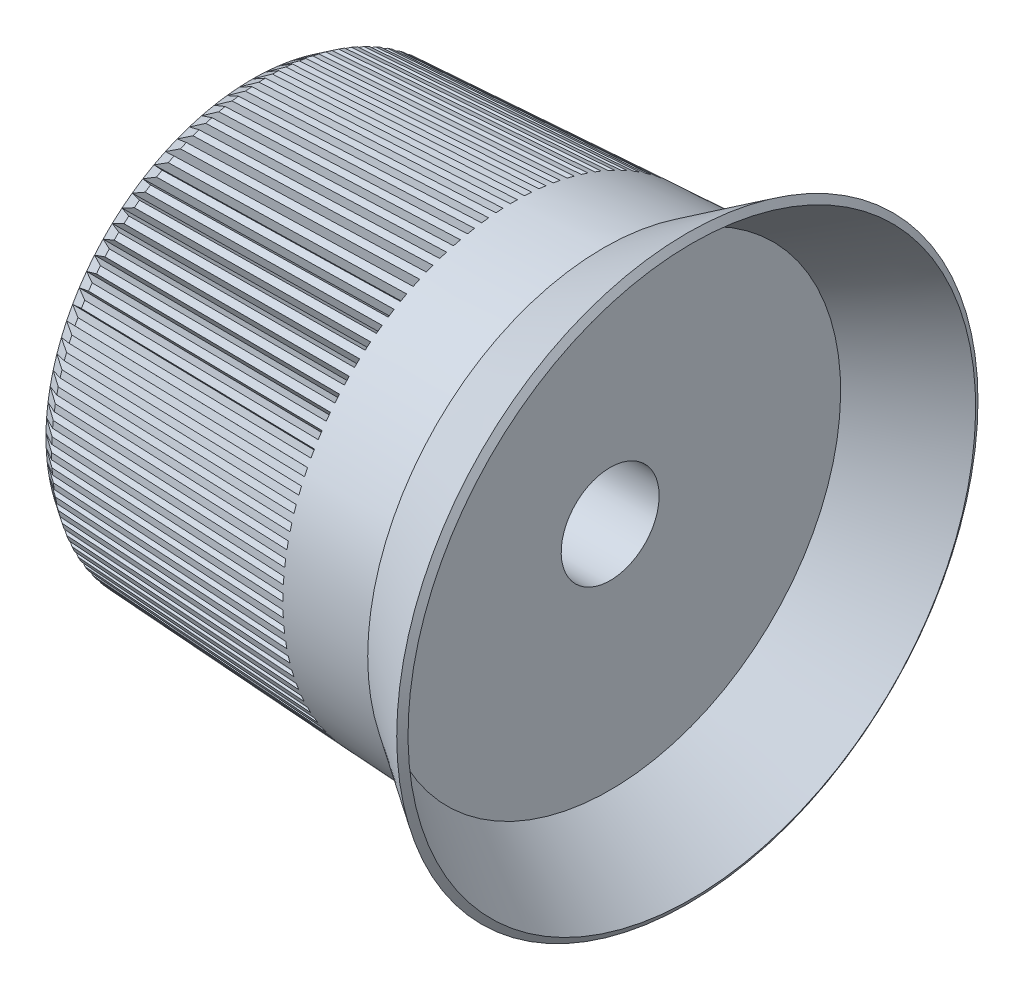
from build123d import *

# Parameters (mm, degrees)
CHAMFER1_SIZE      = 2
CHAMFER1_SIZE2     = 1.195005807
CIRPATTERN1_COUNT  = 101
SKETCH4_R          = 3
CUT_EXTRUDE1_DEPTH = 90


with BuildPart() as part:
    # Sketch1 → Revolve1 (revolve)
    with BuildSketch(Plane.XY):
        Polygon((0, 0), (0, 26.5), (43, 28.9), (53.252971779, 35.6), (53.8, 34.762885835), (43.8, 28.22819507), (43.8, 6), (3.8, 6), (3.8, 0), align=None)
    revolve(axis=Axis((3.8, 0, 0), (-1, 0, 0)))

    # Chamfer1
    chamfer1_edges = [part.edges().sort_by_distance(p)[0] for p in [
        (0, -26.5, 0),
    ]]
    chamfer1_side = [part.faces().sort_by_distance(p)[0] for p in [
        (21.5, -27.7, 0),
    ]]
    chamfer(chamfer1_edges, length=CHAMFER1_SIZE, length2=CHAMFER1_SIZE2, reference=chamfer1_side[0])

    # Cut-Sweep1: sweep along a path in Sketch3
    with BuildLine(Plane.XY) as cut_sweep1_path:
        Line((0, 25.304994193), (32, 27.091040704))
    # Sketch2 → Cut-Sweep1 (sweep, cut)
    with BuildSketch(Plane.ZY):
        Polygon((0, 25.304994193), (1.819851171, 30.304994193), (-1.819851171, 30.304994193), align=None)
    cut_sweep1 = sweep(path=cut_sweep1_path.line, mode=Mode.SUBTRACT)

    # CirPattern1: Cut-Sweep1 ×101 about axis
    cirpattern1_axis = Axis((0, 0, 0), (1, 0, 0))
    for i in range(1, CIRPATTERN1_COUNT):
        add(cut_sweep1.rotate(cirpattern1_axis, i * 360 / CIRPATTERN1_COUNT), mode=Mode.SUBTRACT)

    # Sketch4 → Cut-Extrude1 (cut)
    with BuildSketch(Plane(origin=(0, 0, 0), x_dir=(1, 0, 0), z_dir=(0, 1, 0))):
        with Locations(Location((25.8, 0, 0), (0, 0, 270))):
            Circle(SKETCH4_R)
    extrude(amount=-CUT_EXTRUDE1_DEPTH, mode=Mode.SUBTRACT)


solid = part.part
